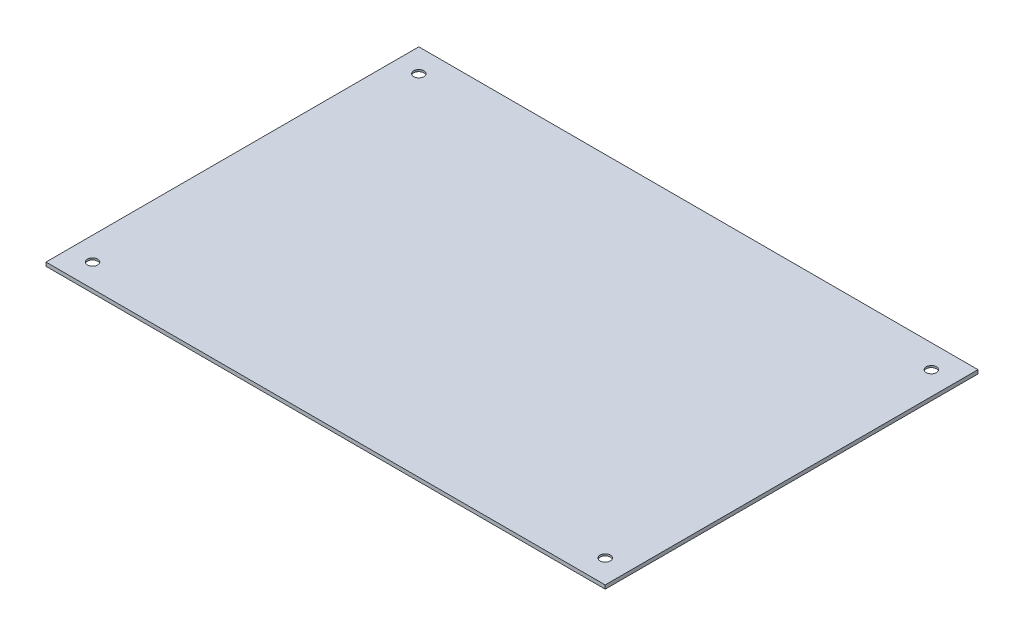
SolidWorks part; units mm, degrees
ref_plane "Front Plane" through (0, 0, 0) normal (0, 0, 1) x (1, 0, 0)
ref_plane "Top Plane" through (0, 0, 0) normal (0, 1, 0) x (1, 0, 0)
ref_plane "Right Plane" through (0, 0, 0) normal (1, 0, 0) x (0, 0, -1)
sketch "Sketch1" plane through (0, 0, 0) normal (0, 1, 0) x (1, 0, 0)
  line L1 (-300, 200) -> (300, 200)
  line L2 (-300, 200) -> (-300, -200)
  line L3 (-300, -200) -> (300, -200)
  line L4 (300, 200) -> (300, -200)
  line L5 (-300, 200) -> (300, -200) construction
  line L6 (-300, -200) -> (300, 200) construction
  point P0 (0, 0)
  dimension "D1" = 600
  dimension "D2" = 400
extrude "Boss-Extrude1" add sketch "Sketch1" along normal blind 4
shell "Shell1" thickness 2
sketch "Sketch2" plane through (0, 4, 0) normal (0, 1, 0) x (1, 0, 0)
  circle A0 centre (-275, 175) radius 5.5
  circle A1 centre (275, 175) radius 5.5
  circle A2 centre (275, -175) radius 5.5
  circle A3 centre (-275, -175) radius 5.5
  dimension "D1" = 11
extrude "Cut-Extrude1" cut sketch "Sketch2" against normal blind 4
